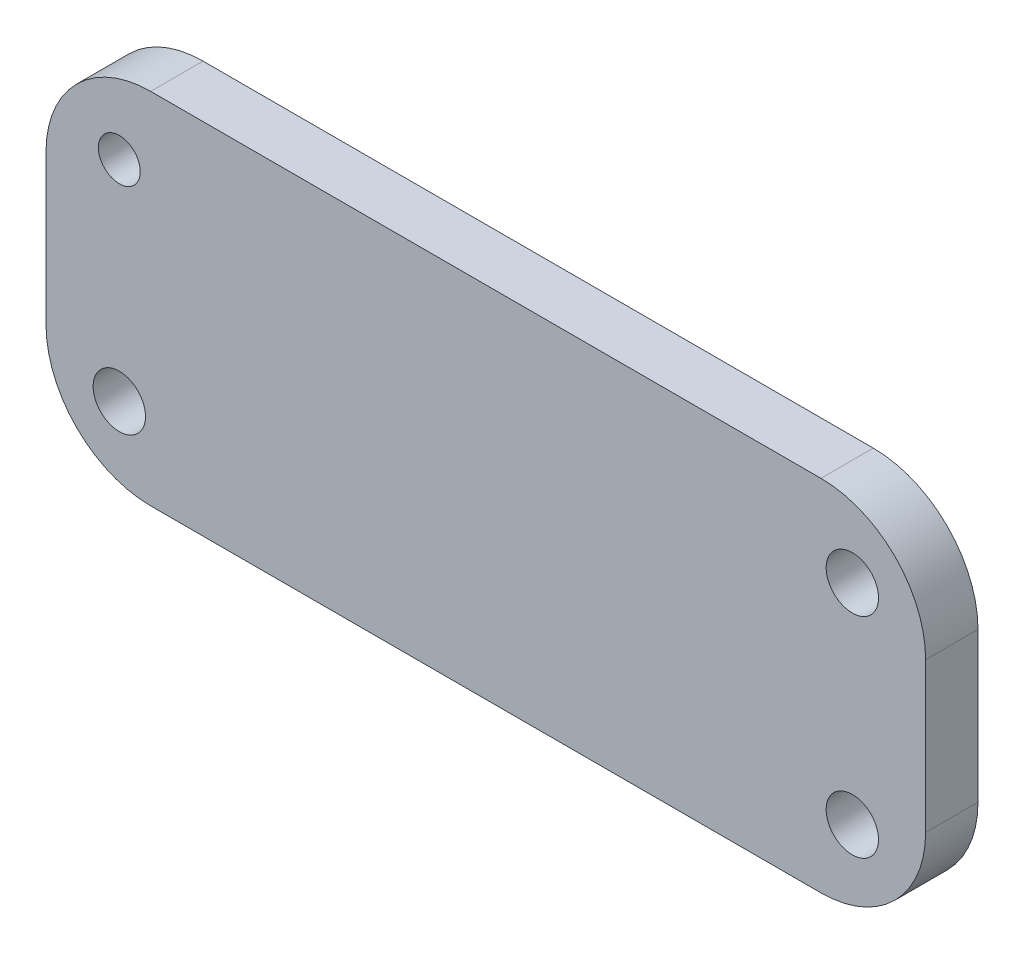
SolidWorks part; units mm, degrees
ref_plane "前视基准面" through (0, 0, 0) normal (0, 0, 1) x (1, 0, 0)
ref_plane "上视基准面" through (0, 0, 0) normal (0, 1, 0) x (1, 0, 0)
ref_plane "右视基准面" through (0, 0, 0) normal (1, 0, 0) x (0, 0, -1)
sketch "草图1" plane through (0, 0, 0) normal (0, 0, 1) x (1, 0, 0)
  line L0 (80, -80) -> (-80, -80) construction
  line L1 (80, -100) -> (80, -60) construction
  line L2 (-80, -60) -> (-80, -100) construction
  line L4 (84, -45.7171) -> (-84, -45.7171)
  line L5 (84, -45.7171) -> (84, -114.2829)
  line L6 (84, -114.2829) -> (-84, -114.2829)
  line L7 (-84, -45.7171) -> (-84, -114.2829)
  line L8 (84, -45.7171) -> (-84, -114.2829) construction
  line L9 (84, -114.2829) -> (-84, -45.7171) construction
  arc A1 (-90, -100) -> (-50, -100) centre (-70, -100) ccw construction
  point P6 (0, -80)
  dimension "D1" = 68.5657
  dimension "D2" = 168
extrude "凸台-拉伸1" add sketch "草图1" against normal blind 10
sketch "草图2" plane through (0, 0, 0) normal (0, 0, 1) x (1, 0, 0)
  circle A0 centre (-70, -60) radius 4
  circle A1 centre (-70, -100) radius 5
  circle A2 centre (70, -60) radius 5
  circle A3 centre (70, -100) radius 5
  dimension "D1" = 8
  dimension "D2" = 10
  dimension "D3" = 10
  dimension "D4" = 10
extrude "切除-拉伸1" cut sketch "草图2" against normal blind 10
fillet "圆角1" radius 20 4 edges at (-84, -45.7171, -5) (84, -45.7171, -5) (84, -114.2829, -5) (-84, -114.2829, -5)
